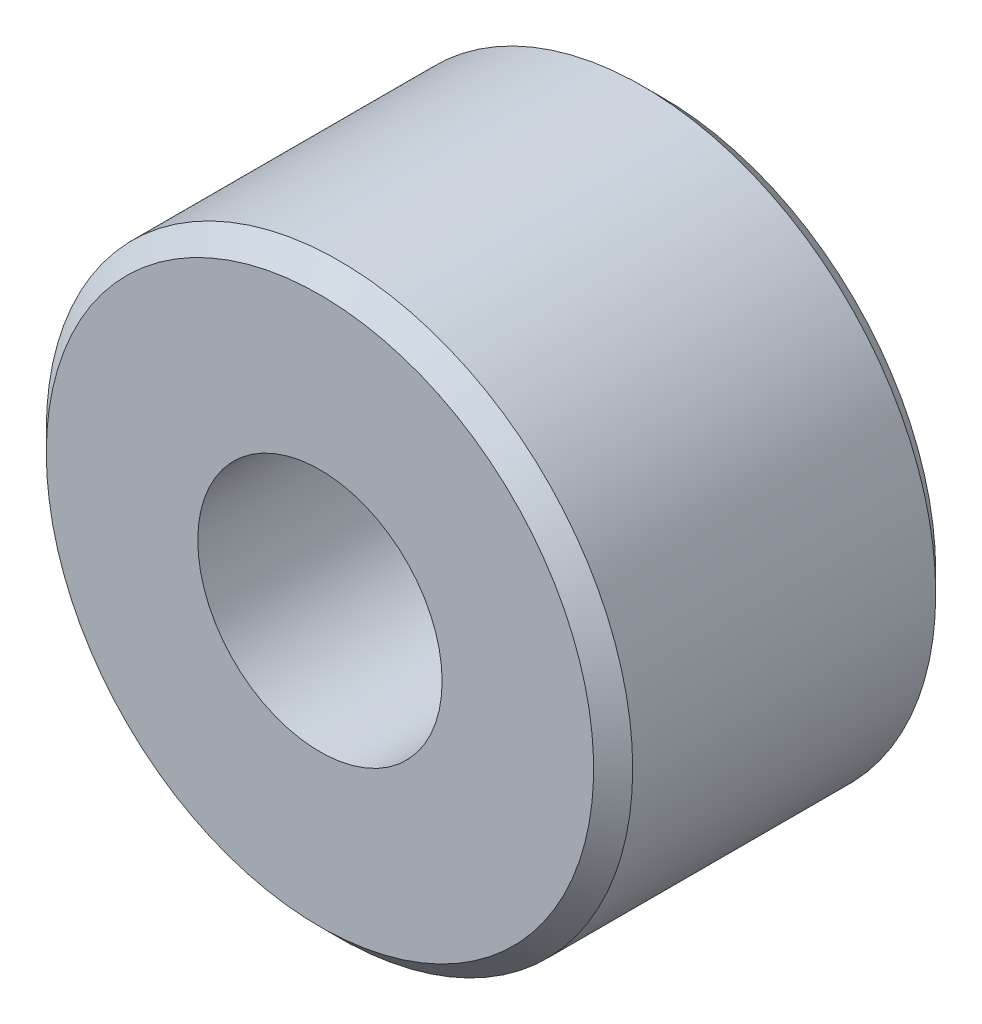
SolidWorks part; units mm, degrees
material "镀铬棒"
ref_plane "Front Plane" through (0, 0, 0) normal (0, 0, 1) x (1, 0, 0)
ref_plane "Top Plane" through (0, 0, 0) normal (0, 1, 0) x (1, 0, 0)
ref_plane "Right Plane" through (0, 0, 0) normal (1, 0, 0) x (0, 0, -1)
sketch "Sketch1" plane through (0, 0, 0) normal (0, 0, 1) x (1, 0, 0)
  circle A0 centre (0, 0) radius 3
  dimension "D1" = 6
extrude "Boss-Extrude1" add sketch "Sketch1" along normal blind 3.5
hole_wizard "M3 Tapped Hole1" positions "Sketch3" profile "Sketch2" tap size "M3" standard "Gb"
sketch "Sketch3" plane through (0, 0, 0) normal (0, 0, -1) x (-1, 0, 0)
  point P0 (0, 0)
sketch "Sketch2" plane through (0, 0, 0) normal (1, 0, 0) x (0, 1, 0)
  line L0 (0, 0) -> (0, 7.5)
  line L1 (0, 7.5) -> (1.25, 7.5)
  line L2 (1.25, 7.5) -> (1.25, 0)
  line L5 (1.25, 0) -> (0, 0)
  line L10 (0, 7.5) -> (-1.25, 7.5) construction
  line L11 (0, -6.35) -> (0, 107.95) construction
  dimension "螺纹孔钻头直径" = 2.5
  dimension "螺纹孔钻头深度" = 7.5
  dimension "导头角度" = 180
cosmetic thread "Cosmetic Thread 1" parameters "D1"=5, "D2"=3
chamfer "Chamfer1" distance 0.2 angle 45 2 edges at (3, 0, 0) (3, 0, 3.5)
